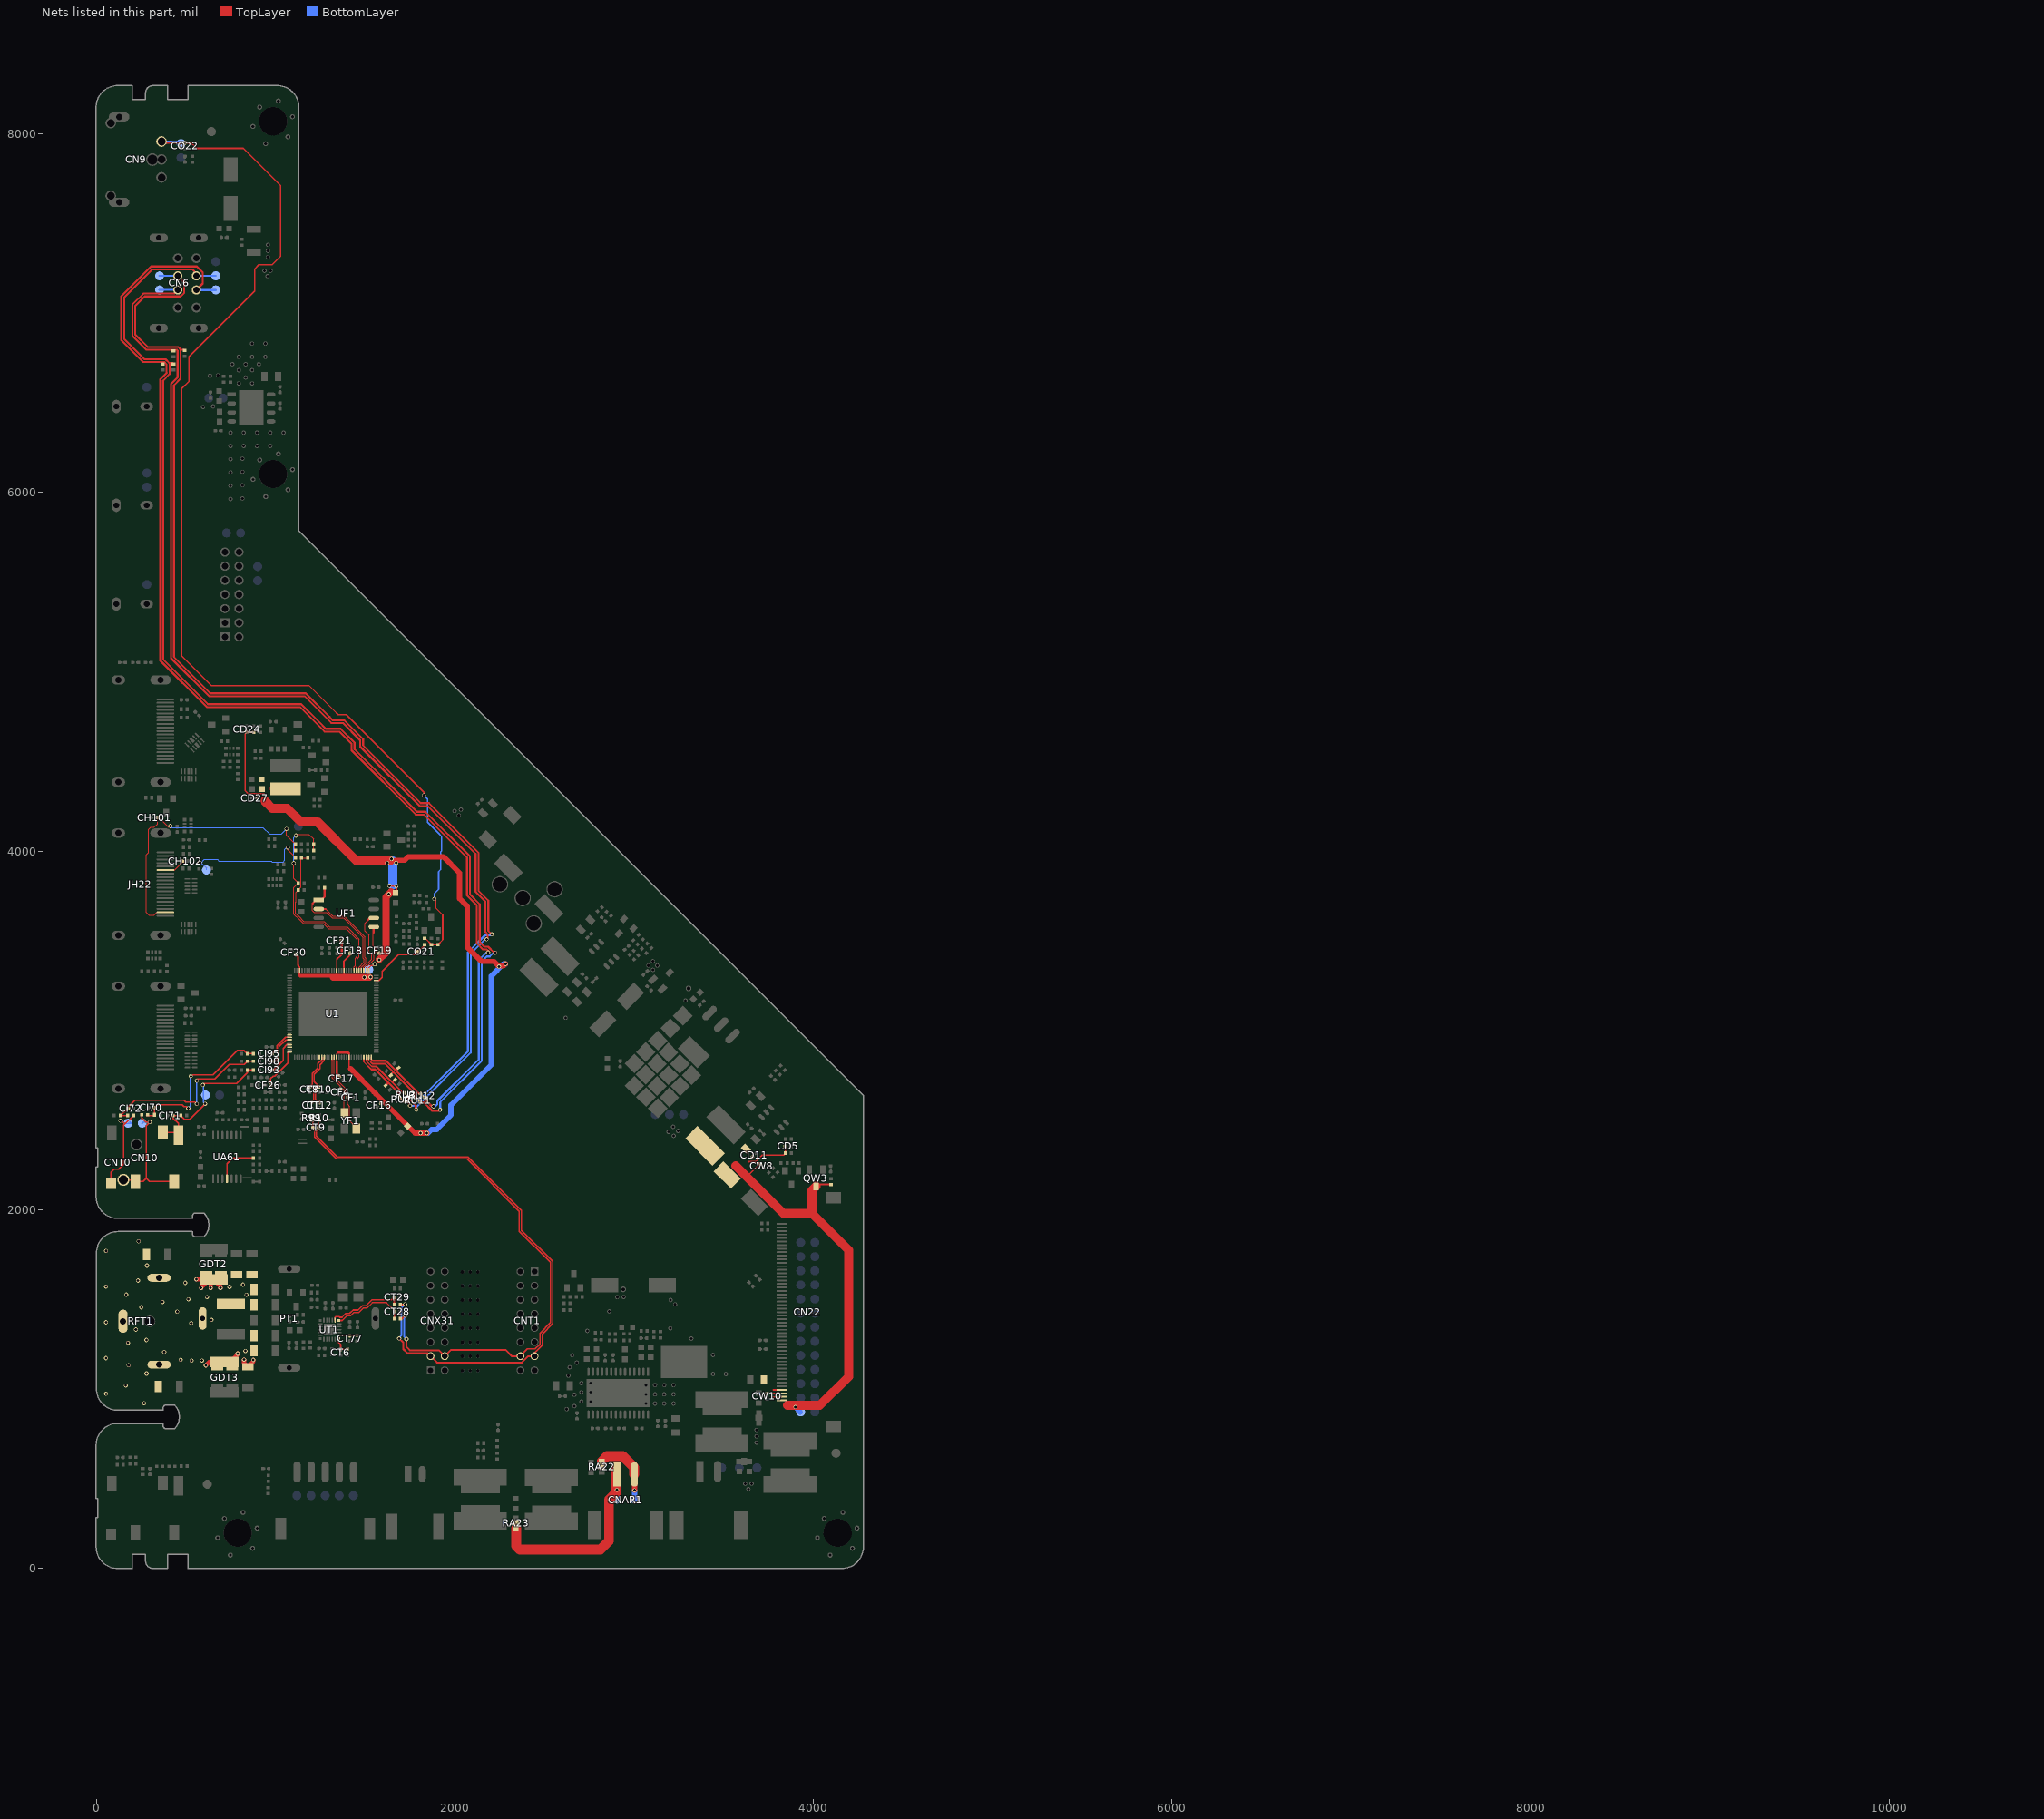
[diagram p0: the nets of this part, all layers, seen from the top]
# Altium PCB MISC105950.PcbDoc (part 13 of 15)
Units mil, origin at the board's own origin, x right, y up, seen from the top; angles counter-clockwise.
Board outline 4280.62 x 8272.76 mil, 2 copper layers (TopLayer, BottomLayer), stack 61.855 mil thick; 541 components, 268 nets, 2324 pads, 1157 vias.

## Via types
v1: diameter 23.62, hole 15.75, TopLayer to BottomLayer, tented both sides, 1087 vias
v2: diameter 23.62, hole 15.75, TopLayer to BottomLayer, 51 vias
v3: diameter 27.56, hole 19.68, TopLayer to BottomLayer, 15 vias
v4: diameter 31.5, hole 19.68, TopLayer to BottomLayer, tented both sides, 4 vias

## Nets (pads, with @x,y where several pads share a name; then routed paths per layer and width w, separated by ;. In a path a pad name is that pad's centre, name@x,y a point inside that pad or via, vN(x,y) a via of type N, cw(c..) or ccw(c..) an arc to the next point about the centre after c; other vN are vias at no path point) (continued)
RFGND: CT41.2 CT42.2 CT43.2 CT44.2 CT45.1 CT46.1 CT47.1 CT48.1 CT49.1 CT50.1 CT51.1 CT52.1 CT53.1 GDT1.2 GDT2.1@613,1635.93 GDT2.1@653,1610.33 GDT2.1@693,1635.96 GDT3.1@674.5,1123.04 GDT3.1@714.5,1148.67 GDT3.1@754.5,1123.07 PT1.1 RFT1.2 RFT1.3 RFT1.4 | length 611.8
  TopLayer w24: v2(556.33,1610.33) GDT2.1@653,1610.33 ; v2(583,1562.5) 583,1564 629.33,1610.33 GDT2.1@653,1610.33 ; v2(609.5,1130) 628.17,1148.67 GDT3.1@714.5,1148.67 743.17,1148.67 787.5,1193 v2(787.5,1196.5) ; v2(636,1562.5) 636,1593.33 GDT2.1@653,1610.33 ; v2(691,1562.5) 691,1572.33 GDT2.1@653,1610.33 ; v2(822.5,1162.5) 822.5,1144.55 CT44.2@844.08,1122.97 874,1152.88 v2(874,1160.5)
  other v1: 264.61,919.44 52.5,971.5 163,1018.5 278.5,1085 178.5,1131.5 529.5,1157 588,1157.5 469,1161.5 52.5,1171 377,1205 830.5,1210.5 175.5,1256 278,1272 219,1330.5 528,1366 52.5,1370.5 641,1384 450,1430.5 250,1454.5 368,1484 511.9,1499.2 616,1511.8 836,1524.5 165.5,1524.8 741.4,1567.9 52.5,1570 816.6,1580.5 494.5,1591 231,1603.95 281,1687.5 52.5,1769.5 234.5,1822.5
ROUT+: CNAR1.1 RA23.2 RA23.3 ROUT+.1 | length 1114.9
  TopLayer w55: RA23.2@2341,220.44 2341,122.5 2360.5,103 2810.5,103 2858.5,151 2858.5,381 2900.65,423.15 CNAR1.1@2900.65,553.5
  BottomLayer w30: v1(2902.5,435.5) 2902.5,384.07 ROUT+.1@2902.57,384
ROUT-: CNAR1.2 RA22.2 RA22.3 ROUT-.1 | length 395.8
  TopLayer w30: v1(3000.71,433.71) CNAR1.2@3000.71,522.37
  TopLayer w55: RA22.2@2818,594.78 2846.99,623.77 2935.73,623.77 2999,560.5 CNAR1.2@2999,522.37
  BottomLayer w30: v1(3000.71,433.71) 3000.71,384.29 ROUT-.1@3001,384
RXD: CH101.2@332.5,4187.5 CH101.2@339.39,4187.5 JH22.2 RH101.1 RH102.1 | length 1529.6
  TopLayer w5: JH22.2@335.35,3657.48 319.37,3641.5 292.65,3641.5 276.69,3657.46 276.69,3978.85 289.5,3991.66 289.5,4120 302.99,4133.49 321.49,4133.49 339.39,4151.39 CH101.2@339.39,4187.5 ; CH101.2@347.39,4187.5 v1@401.33,4133.56 ; v1(1059.17,4123.81) 1059.17,4088.28 RH102.1@1109.7,4037.75 ; RH101.1@1105.77,4009.75 RH102.1@1105.77,4037.75
  BottomLayer w5: v1(410.88,4139.3) 419.99,4130.19 928.65,4130.19 964.65,4094.19 1030.19,4094.19 1059.17,4123.17 v1(1059.17,4123.81)
SPDIF_OUT: CN9.1 CO22.1 DO21.K RO21.2 RO22.2 SPDIF_OUT.1 | length 6462
  TopLayer w8: CO22.1@493.5,7952.11 497.71,7947.89 530.92,7947.89 558.31,7920.5 818.97,7920.5 1026.5,7712.97 1026.5,7318.16 979.45,7271.11 956.5,7271.11 956.38,7271 950.62,7271 905.22,7271.01 882,7247.79 882,7124.5 515,6757.5 515,6620 475,6580 475,5087.9 639.4,4923.5 1185.12,4923.5 1324.06,4784.56 1347.62,4761 1393.31,4761 1826,4328.31 v1(1826,4310) ; RO21.2@1830,3511.73 1834.53,3511.73 1868.5,3477.77 RO22.2@1904.5,3477.77 ; v1(1884.5,3732.5) 1890.5,3726.5 1890.5,3684 1931,3643.5 1931,3504.77 RO22.2@1904.5,3478.27
  TopLayer w10: CN9.1@368.87,7951.61 CO22.1@493.5,7951.61
  BottomLayer w8: v1(1826,4310) 1846,4290 1846,4161 1915,4092 1915,4091.88 1925.31,4081.57 1925.31,3999.68 1919,3993.37 1919,3896.35 1908.31,3885.66 1908.31,3786.31 1884.5,3762.5 v1(1884.5,3732.5)
  BottomLayer w10: CN9.1@360.31,7956.38 CN9.1@362.2,7958.27 459.97,7958.27 SPDIF_OUT.1@470.87,7947.38
SPDIF_OUT_IC: CO21.2@1794.26,3438.5 CO21.2@1801.15,3438.5 RO21.1 U1.94 | length 402.6
  TopLayer w7: U1.94@1560.66,3277.9 1574.83,3277.9 1592.94,3296 1592.94,3328.99 1685.44,3421.5 1728,3421.5 ; 1699.44,3421.5 1728,3421.5 ; RO21.1@1830,3478.27 1830,3474.24 CO21.2@1794.26,3438.5 1777.26,3421.5 1728,3421.5
SPI_CLK: U1.100 UF1.6 | length 360.1
  TopLayer w5: U1.100@1490.74,3334.04 1490.74,3351.4 1535.31,3395.97 1535.31,3421.5 1519.31,3437.5 1519.31,3531.16 1496.56,3553.91 1496.56,3597.56 1511.75,3612.75
  TopLayer w12: 1511.75,3612.75 1525.5,3626.5 UF1.6@1546.59,3626.5
SPI_CSN: RF3.1 U1.102 UF1.1 | length 744.2
  TopLayer w5: 1204.22,3709.72 1202.47,3707.97 1202.47,3668.5 1213.78,3657.19 1283.03,3657.19 1314.29,3625.93 1377.5,3625.93 1486.31,3517.12 1486.31,3401.5 1491.43,3396.37 1491.43,3380.38 1463.19,3352.13 U1.102@1463.19,3334.04 ; 1271.73,3758.73 RF3.1@1271.73,3795.5
  TopLayer w12: 1205.97,3707.97 UF1.1@1228.23,3730.23 ; UF1.1@1239.5,3726.5 1253.5,3726.5 1271.73,3744.73 RF3.1@1271.73,3795.5
SPI_DI: U1.99 UF1.5 | length 272.1
  TopLayer w5: U1.99@1504.52,3334.04 1504.52,3351.04 1548.5,3395.02 1548.5,3427.69 1558.31,3437.5 1558.31,3453.5 1542.31,3469.5 1542.31,3546 ; UF1.5@1545.81,3575.72 1546.16,3576.07 UF1.5@1546.16,3576.5
  TopLayer w12: 1545.81,3546 UF1.5@1545.81,3575.72 ; UF1.5@1546.16,3576.07 UF1.5@1546.59,3576.5
SPI_DO: U1.101 UF1.2 | length 540.8
  TopLayer w5: 1277.86,3676.5 1318.43,3635.93 1381.64,3635.93 1402.6,3614.97 1402.97,3614.97 1496.31,3521.63 1496.31,3405.64 1501.43,3400.52 1501.43,3376.23 1476.96,3351.77 U1.101@1476.96,3334.04
  TopLayer w12: UF1.2@1219.5,3676.5 UF1.2@1239.5,3676.5 1277.86,3676.5
TUNER_AGC_OUT_IC: U1.43
TUNER_IF_N_IN: CT29.1 RT5.1 UT1.14 | length 444.2
  TopLayer w7: UT1.14@1331,1383.15 1331,1397 1336,1402 1351.79,1402 1355.1,1398.69
  TopLayer w8: 1355.1,1398.69 1369.87,1398.69 1391.18,1420 1411.68,1420 1430.68,1439 1459.18,1439 1483.29,1463.11 1503.1,1463.11 1536,1496 1596,1496 ; 1611.5,1496 1596,1496 ; 1642.77,1496 1596,1496 ; 1646.27,1496.5 CT29.1@1660.27,1510.5 RT5.1@1660.27,1471
TUNER_IF_N_IN_CN: CNT1.13 CNX31.3 CT9.1 R10.2 R10.3 RT5.2 | length 3408.3
  TopLayer w7: R10.2@1244,2495.04 1240.07,2491.11 CT9.1@1240.07,2457 1240.07,2450.07 1227,2437 1227,2409.52 1342.52,2294 2070.56,2294 2370.5,1994.06 2370.5,1883.97 2544.5,1709.97 2544.5,1363.85 2485.36,1304.72 2485.36,1242.95 2443.21,1200.79 CNT1.13@2443.21,1181.67 CNT1.13@2445.14,1181.67
  TopLayer w10: v1(1688,1280.5) 1711,1257.5 1711,1221.5 1733,1199.5 1845.44,1199.5 CNX31.3@1863.21,1181.73 1898.94,1146 2373.57,1146 2409.24,1181.67 CNT1.13@2443.21,1181.67 ; RT5.2@1694.23,1470.5 1720.27,1470.5 v1(1720.9,1471.14)
  BottomLayer w10: v1@1690,1285.88 1700.5,1296.38 1700.5,1450.73 v1(1720.9,1471.14)
TUNER_IF_N_IN_IC: CT10.1 CT12.1 U1.45 | length 314.6
  TopLayer w7: CT12.1@1244,2593.46 1222.31,2615.15 1222.31,2675 1233.54,2686.23 CT10.1@1241,2686.23 1214.5,2712.73 1214.5,2754.94 1245.37,2785.82 1245.37,2807.82 1270.27,2832.71 U1.45@1270.27,2849.72 ; CT12.1@1246.25,2595.71 CT12.1@1248.5,2593.46
TUNER_IF_P_IN: CT28.2@1661.26,1431.5 CT28.2@1668.15,1431.5 RT4.1 UT1.13 | length 418.5
  TopLayer w8: UT1.13@1350.48,1381 1370.56,1381 1396.56,1407 1417.06,1407 1436.06,1426 1464.56,1426 1488.67,1450.11 1508.49,1450.11 1538.38,1480 1617.59,1480 1661.26,1436.32 CT28.2@1661.26,1431.5 ; CT28.2@1657,1431.5 CT28.2@1661.26,1431.5 ; RT4.1@1661.26,1392.01 CT28.2@1661.26,1431.5
TUNER_IF_P_IN_CN: CNT1.14 CNX31.4 CT9.2@1206.61,2457 CT9.2@1213.5,2457 R99.2 R99.3 RT4.2 | length 3294.4
  TopLayer w7: R99.2@1201.5,2495.04 1206.61,2489.92 CT9.2@1206.61,2457 1206.61,2449.78 1215,2441.39 1215,2404.55 1337.55,2282 2065.59,2282 2358.5,1989.09 2358.5,1879 2532.5,1705 2532.5,1368.82 2473.36,1309.69 2473.36,1247.92 2446.95,1221.5 2404.3,1221.5 CNT1.14@2364.47,1181.67
  TopLayer w10: RT4.2@1695.23,1391.5 1705.28,1391.5 v1(1722.31,1408.53) ; v1(1729,1277) 1729,1232 1746.5,1214.5 1909.18,1214.5 CNX31.4@1941.95,1181.73 1977.22,1217 2280.5,1217 2315.83,1181.67 CNT1.14@2364.47,1181.67
  BottomLayer w7: v1@1725,1277 v1(1729,1277)
  BottomLayer w10: v1(1722.31,1408.53) 1715.5,1401.72 1715.5,1290.5 v1(1729,1277)
TUNER_IF_P_IN_IC: CT1.1 CT8.2@1189,2679.35 CT8.2@1189,2686.24 U1.44 | length 306.7
  TopLayer w7: CT8.2@1189,2683.49 1202.5,2696.99 1202.5,2758.5 1234.37,2790.37 1234.37,2813.79 1256.49,2835.91 U1.44@1256.49,2849.72 ; CT8.2@1189,2686.24 1197.76,2686.24 1210.31,2673.69 1210.31,2600.17 CT1.1@1201.5,2591.35
TUNER_SCL_OUT: CT6.2@1361.5,1213.35 CT6.2@1361.5,1220.24 RT2.2 UT1.7 | length 104.8
  TopLayer w8: UT1.7@1350.5,1280.02 UT1.7@1350.5,1279.02 1350.5,1258.5 1361.5,1247.5 CT6.2@1361.5,1221.23 ; CT6.2@1360.5,1221.23 CT6.2@1361.5,1221.23 ; CT6.2@1361.5,1220.24 CT6.2@1361.5,1221.23 ; RT2.2@1401,1221.23 CT6.2@1361.5,1221.23
TUNER_SDA_IO: CT77.2@1412.5,1291.35 CT77.2@1412.5,1298.24 RT3.2 UT1.8 | length 99.4
  TopLayer w7: UT1.8@1352.65,1298.5 RT3.2@1451.77,1298.5
  TopLayer w8: RT3.2@1451.77,1298.5 RT3.2@1452,1298.73
TXD: CH102.2@477.1,3943.6 CH102.2@483.99,3943.6 JH22.14 RH103.1 TXD.1 | length 967.6
  TopLayer w5: JH22.14@384.16,3893.7 433.7,3893.7 481,3941 498.67,3923.33 518,3923.33 ; 560.5,3923.33 518,3923.33 ; v1(576.5,3935.5) 564.33,3923.33 518,3923.33 ; v1@1059.5,4019.5 v1(1067,4019.5) 1067,4006.28 1110.2,3963.08 RH103.1@1110.2,3961.25
  BottomLayer w5: TXD.1@613,3894 613,3905 584,3934 602.31,3952.31 673.5,3952.31 683,3942.81 974.69,3942.81 978.07,3939.43 1041,3939.43 1049.16,3947.58 1049.16,4009.16 1059.5,4019.5 v1(1067,4019.5)
UART_RX_IC: CD101.K RH105.2 RH106.1 U1.104 | length 1241.5
  TopLayer w5: v1(1100,3931.5) 1098.5,3930 1098.5,3846.77 CD101.K@1124.27,3821 1101,3797.73 1101,3646.94 1129.31,3618.64 1129.52,3618.64 1152.35,3595.81 1265.22,3595.81 1294.72,3566.31 1393.28,3566.31 1455.31,3504.28 1455.31,3414.09 1442.81,3401.59 1442.81,3360.5 1435.63,3353.32 U1.104@1435.63,3334.04 ; v1(1112,4086) 1119.5,4093.5 1184.5,4093.5 1210.66,4067.34 RH105.2@1210.66,4037.75 RH106.1@1210.66,4002
  BottomLayer w5: v1(1100,3931.5) 1100,4074 v1@1110,4084 ; v1@1110,4084 1110,4088 v1(1112,4086) v1@1110,4084
UART_TX_IC: CD102.K RH103.2 RH104.1 U1.103 | length 951.6
  TopLayer w5: RH103.2@1141.37,3958.97 1141.37,3800.11 CD102.K@1124.27,3783 1111.19,3769.92 1111.19,3715.19 1111,3715 1111,3651.09 1123.65,3638.44 1123.86,3638.44 1156.49,3605.81 1269.36,3605.81 1298.86,3576.31 1397.43,3576.31 1465.31,3508.43 1465.31,3409.94 1452.81,3397.44 1452.81,3356.36 1449.41,3352.95 U1.103@1449.41,3334.04 U1.103@1451.35,3335.98 ; RH103.2@1143.66,3961.25 RH104.1@1177.7,3961.25
USB0_DM_IO: CN6.2 DM0.1 DU11.K RU11.2 RU11.3 | length 6766.8
  TopLayer w11: DU11.K@429.5,6718.11 425.91,6721.7 406.67,6721.7 ; CN6.2@556.3,7208.67 556.3,7223.96 535.5,7244.76 310.11,7244.76 154.5,7089.14 154.5,6856.13 266.63,6744 384.38,6744 406.67,6721.7 ; RU11.2@1805.87,2597.13 1825.79,2597.13 1873.11,2549.81 v1@1910.55,2549.81 ; v1(2224,3432) 2218.5,3432 2184,3466.5 2162.62,3466.5 2137.72,3491.4 2137.72,3523.14 2137.72,3703.54 2082.5,3758.76 2082.5,3970.5 1833.5,4219.5 1787.25,4219.5 1438.5,4568.25 1438.5,4604.79 1360.79,4682.5 1278.33,4682.5 1238.67,4722.17 1141.83,4819 621.57,4819 370.5,5070.07 370.5,6624.12 407,6660.62 407,6721.38 406.67,6721.7
  BottomLayer w11: CN6.2@557.01,7209.38 CN6.2@556.3,7208.67 664.16,7208.67 DM0.1@664.87,7209.38 ; v1(1916.86,2556.12) 1916.86,2598.96 2148.45,2830.55 2148.45,3383.45 2176.5,3411.5 2193.3,3411.5 v1@2213.8,3432
USB0_DM_IO_IC: DU31.K RU11.1 U1.63 | length 397.8
  TopLayer w8: U1.63@1518.3,2849.72 1518.3,2833.2 1537.5,2814
  TopLayer w11: 1539.62,2814 1607.85,2814 1780.77,2641.08 RU11.1@1780.77,2622.23 ; DU31.K@1639.48,2750.52 1655.39,2766.42
USB0_DP_IO: CN6.3 DP0.1 DU12.K RU12.2 RU12.3 | length 6796.3
  TopLayer w11: CN6.3@556.3,7129.93 592.39,7166.02 592.39,7227.99 559.62,7260.76 303.48,7260.76 138.5,7095.77 138.5,6849.5 260,6728 377.75,6728 390.67,6715.08 390.67,6667.57 391,6667.25 354.5,6630.75 354.5,5063.45 614.95,4803 1135.2,4803 1271.7,4666.5 1354.16,4666.5 1422.5,4598.16 1422.5,4561.62 1780.62,4203.5 1826.65,4203.5 2066.5,3963.65 2066.5,3752.13 2121.72,3696.92 2121.72,3529.77 2121.72,3484.77 2155.99,3450.5 2177.37,3450.5 2185.43,3442.44 2185.43,3434.56 2184.37,3433.5 v1(2184.06,3433.81) ; RU12.2@1830.27,2615.27 v1@1870.55,2575
  BottomLayer w11: CN6.3@557.75,7129.93 CN6.3@556.3,7129.93 664.16,7129.93 DP0.1@664.87,7130.64 ; v1@1889.5,2575 1900.86,2586.36 1900.86,2605.59 2132.45,2837.18 2132.45,3390.95 v1@2175.5,3434
  other v1: 1879.5,2575
USB0_DP_IO_IC: DU32.K RU12.1 U1.64 | length 383.6
  TopLayer w8: U1.64@1532.08,2849.72 1532.08,2837.8 1541.38,2828.5
  TopLayer w11: 1542.01,2830 1614.48,2830 1800.84,2643.64 RU12.1@1802.17,2643.64 ; 1669.39,2775.73 DU32.K@1684.33,2790.67
USB1_DM_IO: CN6.6 DM1.1 DU1.K RU2.2 RU2.3 | length 6594.4
  TopLayer w11: CN6.6@453.15,7208.67 489.24,7172.57 489.24,7114.98 468.1,7093.83 268.08,7093.83 215.5,7041.25 215.5,6881.39 284.39,6812.5 454.51,6812.5 468,6799.01 468,6635.35 431.5,6598.85 431.5,5082.61 634.11,4880 1167.1,4880 1299.27,4747.83 1316.6,4730.5 1380.67,4730.5 1486.5,4624.67 1486.59,4624.59 1486.59,4589.18 1808.27,4267.5 1853.64,4267.5 2130.5,3990.64 2130.5,3778.64 2185.72,3723.43 2185.72,3554.35 v1@2204.78,3535.28 ; 470.54,6796.47 DU1.K@487.64,6796.47 ; RU2.2@1714.69,2602.81 1733.84,2602.81 1748.5,2588.15 v1(1748.5,2578.5)
  BottomLayer w11: DM1.1@351.07,7208.88 452.94,7208.88 CN6.6@453.15,7208.67 ; v1(1748.5,2578.5) 1768.05,2578.5 2071.45,2881.89 2071.45,3434.24 2166.78,3529.58 2199.08,3529.58 v1(2205,3535.5)
USB1_DM_IO_IC: DU33.K RU2.1 U1.61 | length 333.3
  TopLayer w8: U1.61@1490.74,2849.72 1490.74,2823.99 1532.73,2782 1534.85,2782
  TopLayer w11: 1534.85,2782 1554.12,2782 1691.03,2645.09 RU2.1@1691.03,2633 ; DU33.K@1612.67,2691.83 1627.55,2706.71
USB1_DP_IO: CN6.7 DP1.1 DU2.K RU3.2 RU3.3 | length 6459.8
  TopLayer w11: CN6.7@453.15,7129.93 433.06,7109.83 261.46,7109.83 199.5,7047.88 199.5,6874.77 277.77,6796.5 447.88,6796.5 452,6792.38 452,6641.98 415.5,6605.48 415.5,5075.99 627.49,4864 1160.47,4864 1309.97,4714.5 1374.05,4714.5 1470.5,4618.05 1470.5,4582.64 1801.64,4251.5 1846.75,4251.5 2114.5,3983.75 2114.5,3772.01 2169.72,3716.8 2169.72,3547.73 2181.04,3536.4 2181.04,3511.24 v1@2176.03,3506.22 ; RU3.2@1740.21,2628.33 1740.21,2619.07 1780.5,2578.78 v1@1780.5,2558.11 ; v1@2175.5,3506.75 v1@2176.03,3506.22 ; v1(2176.03,3507.27) v1@2176.03,3506.22
  BottomLayer w11: DP1.1@351.07,7130.14 452.94,7130.14 CN6.7@453.15,7129.93 ; v1(1782.42,2556.19) 1782.42,2570.24 2087.45,2875.27 2087.45,3426.77 v1@2167.95,3507.27
USB1_DP_IO_IC: DU34.K RU3.1 U1.62 | length 319.6
  TopLayer w8: U1.62@1504.52,2849.72 1504.52,2828.59 1536.18,2796.94
  TopLayer w11: 1537.24,2798 1560.74,2798 1706.75,2651.99 RU3.1@1712,2651.99 ; 1652.13,2711.29 DU34.K@1665.17,2724.33
UVP: RA72.2 UA61.11 | length 245.4
  TopLayer w8: UA61.11@727.18,2171.5 727.18,2254.68 760,2287.5 RA72.2@875.77,2287.5
VCC_PANEL: CD5.2@3841.54,2353.5 CD5.2@3848.43,2353.5 CD11.2@3657.67,2291.67 CD11.2@3662.54,2296.54 CD99.1 CN22.1 CN22.2 CN22.3 CN22.4 CW8.1 CW9.2 CW10.2@3741.5,968.85 CW10.2@3741.5,975.74 ED6.1 LD1.2 QW3.D RD31.2 RW11.2 VCC_PANEL1.1 | length 2697
  TopLayer w8: 3634.55,2189.43 CW8.1@3698.92,2253.8 ; 3639,2266.48 3677.48,2266.48 3714,2303 3832.56,2303 3844.1,2314.54 3844.1,2352.93 CD5.2@3843.54,2353.5 ; 3777.25,954.91 CN22.2@3823.43,954.91
  TopLayer w9: 3770.59,974.59 CN22.3@3823.43,974.59 ; 3776.28,994.28 CN22.4@3823.43,994.28
  TopLayer w10: QW3.D@4023.88,2139.27 RW11.2@4097.5,2139.27
  TopLayer w50: 3566.5,2243 3831,1978.5 3991,1978.5 4195.5,1774 4195.5,1067.5 4035,907 3855,907 ; 3991.5,1994.5 3991.5,2106.88 QW3.D@4013.84,2129.22
  BottomLayer w7: VCC_PANEL1.1@3925.74,870.76 VCC_PANEL1.1@3928.5,870.76
  BottomLayer w30: v1(3898.5,898) VCC_PANEL1.1@3925.74,870.76
VCOM0: CF26.1 U1.32 | length 238.2
  TopLayer w7: CF26.1@975.73,2694 970,2699.73 970,2729.55 971.77,2731.32 985.17,2744.72 992.96,2744.72 1066.06,2817.82 1066.06,2873.06 1071.29,2878.29 U1.32@1076.34,2878.29
VDDC_CORE: CD24.2@838,4663.76 CD24.2@838,4670.65 CD25.2 CD26.2 CD27.2@892,4295.5 CD27.2@898.89,4295.5 CF15.2 CF16.2@1582.92,2588.42 CF16.2@1587.79,2593.29 CF17.2@1353.67,2743.33 CF17.2@1358.54,2738.46 CF18.1 CF19.1 CF20.2@1106.63,3427.37 CF20.2@1111.5,3422.5 CF21.1 CF59.2 LD21.1 pad.VIA5@1494,3295.26 pad.VIA5@1528,3297 pad.VIA5@1551.5,3368.5 pad.VIA5@1576.5,3392.5 pad.VIA5@1621,3933 pad.VIA5@1630.75,3760 pad.VIA5@1634,3806 pad.VIA5@1646,3956 pad.VIA5@1671.5,3933.5 pad.VIA5@1672,3805 pad.VIA5@1807.5,2426.5 pad.VIA5@1842,2426.5 pad.VIA5@2245.12,3355.62 pad.VIA5@2281.5,3370 RD81.2 U1.50 U1.55 U1.98 U1.108 U1.111 U1.126 VCC_CORE.1 | length 6154.9
  TopLayer w8: CD24.2@838,4663.76 CD24.2@837.5,4663.27 ; RD81.2@877,4663.27 838,4663.27 CD24.2@837.5,4663.27 ; 934.84,4320.66 844.41,4320.66 829.65,4335.42 829.65,4655.41 CD24.2@837.5,4663.27 ; 1126.69,3357.94 1132.48,3352.16 U1.126@1132.48,3334.04 1132.48,3308 ; 1339.17,3298.92 U1.111@1339.17,3334.04 1339.61,3334.48 1339.61,3394.61 1340.31,3395.31 ; 1340.16,2823.49 1339.17,2824.48 U1.50@1339.17,2849.72 1339.17,2869.19 1342.49,2872.51 ; 1380.51,3296.26 U1.108@1380.51,3334.04 1380.51,3353.5 ; 1406.28,2871.78 1408.07,2870 U1.55@1408.07,2849.72 1408.07,2819.48 ; 1408.07,2793.77 1408.07,2819.48 ; 1408.07,2809.33 1408.07,2819.48 ; U1.98@1518.3,3334.04 1518.3,3348.56 1530.25,3360.5 1541,3360.5 ; CF19.1@1579.5,3429.27 1592.27,3429.27
  TopLayer w10: 1341.31,3396.31 1363.05,3418.05 ; CF21.1@1361.34,3501.77 CF21.1@1362.57,3503 ; 1380.51,3353.5 1380.51,3386.01 ; 1401.5,3407 1380.51,3386.01 ; CF18.1@1414,3427.77 1414,3419.5 1380.51,3386.01 ; pad.VIA5@1642,3805 pad.VIA5@1672,3805 CF15.2@1672,3766.81
  TopLayer w12: CF20.2@1111.5,3422.5 1123.81,3410.19 1123.81,3363.65 1126.53,3360.93 ; 1362.34,3418.75 1368.89,3425.3 CF21.1@1368.89,3500.5
  TopLayer w15: 1340.16,2823.49 1340.16,2756.84 CF17.2@1353.67,2743.33 ; 1345.98,2876 1402.07,2876 1406.28,2871.78
  TopLayer w20: 1132.48,3308 1135.22,3305.26 1310,3305.26 1320,3295.26
  TopLayer w30: 1418.29,2784.72 1546.5,2656.5 ; 1560,2643.01 1546.5,2656.5 ; 1668,3948.5 1718.47,3948.5 1737.78,3967.81 1934.69,3967.81 2025,3877.5 2025,3734.94 2067,3692.94 2067,3464.94 2147.94,3384 2216.73,3384 2240.92,3359.81 2270.31,3359.81 ; pad.VIA5@1842,2426.5 1776.51,2426.5 1546.5,2656.5 ; pad.VIA5@2249.31,3359.81 2270.31,3359.81 ; pad.VIA5@2281,3370.5 2270.31,3359.81
  TopLayer w40: 1320,3295.26 pad.VIA5@1521.88,3295.26 ; pad.VIA5@1576,3394.79 1614.34,3433.13 1614.34,3512 ; 1614.34,3535.84 1614.34,3512 ; 1643.5,3772 1614.34,3742.84 1614.34,3512
  TopLayer w50: 938,4280.06 979.06,4239 1062.63,4239 1135.63,4166 1228.67,4166 1450.17,3944.5 1638,3944.5 ; LD21.1@990.96,4346.54 LD21.1@1055,4346.54
  BottomLayer w30: pad.VIA5@1812,2426.5 pad.VIA5@1842,2426.5 1849.01,2426.5 1869.2,2446.69 1897.19,2446.69 1977.67,2527.17 1977.67,2582.7 2202.95,2807.98 2202.95,3303.19 2269.75,3370 pad.VIA5@2281.5,3370
  BottomLayer w50: 1653,3809 1653,3945.5
VGA_HS_IN_IC: U1.25
VGA_VS_IN_IC: U1.30
XTAL_IN_IC: CF4.2@1361.5,2665.5 CF4.2@1361.5,2672.39 U1.48 YF1.3 | length 328.7
  TopLayer w5: U1.48@1311.61,2849.72 1311.61,2835.31 1315.16,2831.77 1315.16,2734.32 1361.5,2687.97 CF4.2@1361.5,2672.39 1375.32,2672.39 1380.81,2666.9 1380.81,2560.26 YF1.3@1382.57,2558.5
XTAL_OUT_IC: CF1.2@1400.93,2625 CF1.2@1407.82,2625 U1.49 YF1.1 | length 455.8
  TopLayer w5: 1325.16,2748.84 1325.16,2755.53 ; U1.49@1325.39,2849.72 1325.16,2849.49 1325.16,2755.53 ; YF1.1@1449.5,2452.2 1449.5,2458.5 1411.72,2496.28 1411.72,2575.28 1400.93,2586.07 CF1.2@1400.93,2625 1391.56,2634.37 1391.56,2672.06 1325.16,2738.46 1325.16,2755.53
YPBPR_PB_IN: CN10.3 CN10.5 CNT0.2 RI63.2 YPbPr_Pb.1 | length 739.3
  TopLayer w7: CNT0.2@149.61,2165.42 206.63,2165.42 CN10.3@216.54,2155.51 258.98,2155.51 277.46,2174 ; RI63.2@250.77,2528.5 250.77,2511.23 274,2488 v1(297,2488) ; v1@291.5,2482.5 277.46,2468.46 277.46,2174 ; CN10.5@433.07,2155.51 295.95,2155.51 277.46,2174
  BottomLayer w7: YPbPr_Pb.1@252,2478 261.5,2487.5 v1@297,2487.5
YPBPR_PB_IN_C: CI70.2@314.85,2568.5 CI70.2@321.74,2568.5 DI23.K RI23.2 RI24.1 RI63.1 | length 885.8
  TopLayer w7: RI63.1@282.77,2529.3 277.96,2524.5 DI23.K@320,2524.5 ; DI23.K@321.26,2529 DI23.K@321.77,2528.5 ; DI23.K@321.74,2529.48 CI70.2@321.74,2568.5 338.74,2585.5 477.25,2585.5 488.06,2574.69 500.81,2574.69 v1(511,2564.5) ; 534.37,2751.37 649.18,2751.37 785.15,2887.34 821.16,2887.34 RI23.2@839.5,2869 ; RI23.2@836.76,2869 RI23.2@839.5,2869 ; RI24.1@875.27,2869 RI23.2@839.5,2869
  BottomLayer w7: v1(511,2564.5) 523,2576.5 523,2740 v1(526,2743)
YPBPR_PB_IN_IC: CI95.2@973.34,2869 CI95.2@980.23,2869 U1.26 | length 145
  TopLayer w7: CI95.2@980.23,2869.5 1005.06,2894.33 1005.06,2913.08 1052.96,2960.97 U1.26@1076.34,2960.97
YPBPR_PR_IN: CI71.2@420.84,2524.5 CI71.2@427.73,2524.5 CN10.4 CN10.6 DI24.K RI25.2 RI26.1 YPbPr_Pr.1 | length 894.5
  TopLayer w7: CN10.4@370.08,2431.1 CN10.6@439.96,2431.1 ; CN10.6@456.69,2414.37 456.69,2479.31 427.73,2508.27 CI71.2@427.73,2524.5 DI24.K@469,2524.5 489.5,2504 519.5,2504 v1(605.5,2590) ; v1(593,2695) 601.37,2703.37 655,2703.37 ; 611.5,2703.37 655,2703.37 ; RI25.2@839.5,2778.5 RI25.2@841.5,2778.5 ; RI26.1@875.27,2778.5 RI25.2@841.5,2778.5 ; 655,2703.37 780.1,2703.37 841.5,2764.78 RI25.2@841.5,2778.5
  BottomLayer w7: v1(593,2695) 595,2693 595,2600.5 v1(605.5,2590)
YPBPR_PR_IN_IC: CI93.2@973.34,2778.5 CI93.2@980.23,2778.5 U1.29 | length 195
  TopLayer w7: CI93.2@980.23,2774.5 983.5,2774.5 1041.06,2832.06 1041.06,2898.17 1062.53,2919.63 U1.29@1076.34,2919.63
YPBPR_Y_IN: CN10.1 RI62.2 YPbPr_Y.1 | length 558.6
  TopLayer w7: CN10.1@80.71,2145.67 80.71,2207.71 97.5,2224.5 124,2224.5 151.45,2251.95 151.45,2470.22 158.42,2477.19 ; v1@138.5,2494 141.61,2494 158.42,2477.19 ; RI62.2@205.73,2524.5 158.42,2477.19
  BottomLayer w7: v1@138.5,2494 143,2494 155.5,2481.5 YPbPr_Y.1@175.76,2481.5 ; YPbPr_Y.1@183.5,2491.5 193.5,2481.5 YPbPr_Y.1@175.76,2481.5 ; YPbPr_Y.1@187,2481.5 YPbPr_Y.1@175.76,2481.5
  other v1: 133,2495
YPBPR_Y_IN_C: CI72.2@173.76,2564 CI72.2@180.65,2564 DI34.K RI36.2 RI38.1 RI62.1 | length 1001.2
  TopLayer w7: DI34.K@132.23,2524.5 DI34.K@134.26,2524.5 ; RI62.1@172.27,2524.5 DI34.K@134.26,2524.5 ; CI72.2@173.76,2564 CI72.2@172.27,2562.5 ; v1(558.5,2589.5) 549.31,2598.69 498,2598.69 486.19,2610.5 213,2610.5 172.27,2569.77 CI72.2@172.27,2562.5 ; v1@559,2727.37 659.12,2727.37 740.9,2809.15 823.16,2809.15 RI36.2@841.5,2827.5 RI38.1@875.27,2827.5 ; DI34.K@134.26,2524.5 CI72.2@172.27,2562.5
  BottomLayer w7: v1@559,2590 v1(559,2718.5)
YPBPR_Y_IN_IC: CI98.2@973.34,2827.5 CI98.2@980.23,2827.5 U1.27 | length 180.9
  TopLayer w7: CI98.2@979,2827.5 CI98.2@979.62,2828.11 ; CI98.2@980.23,2827.5 995,2827.5 1017.06,2849.56 1017.06,2908.11 1056.15,2947.19 U1.27@1076.34,2947.19